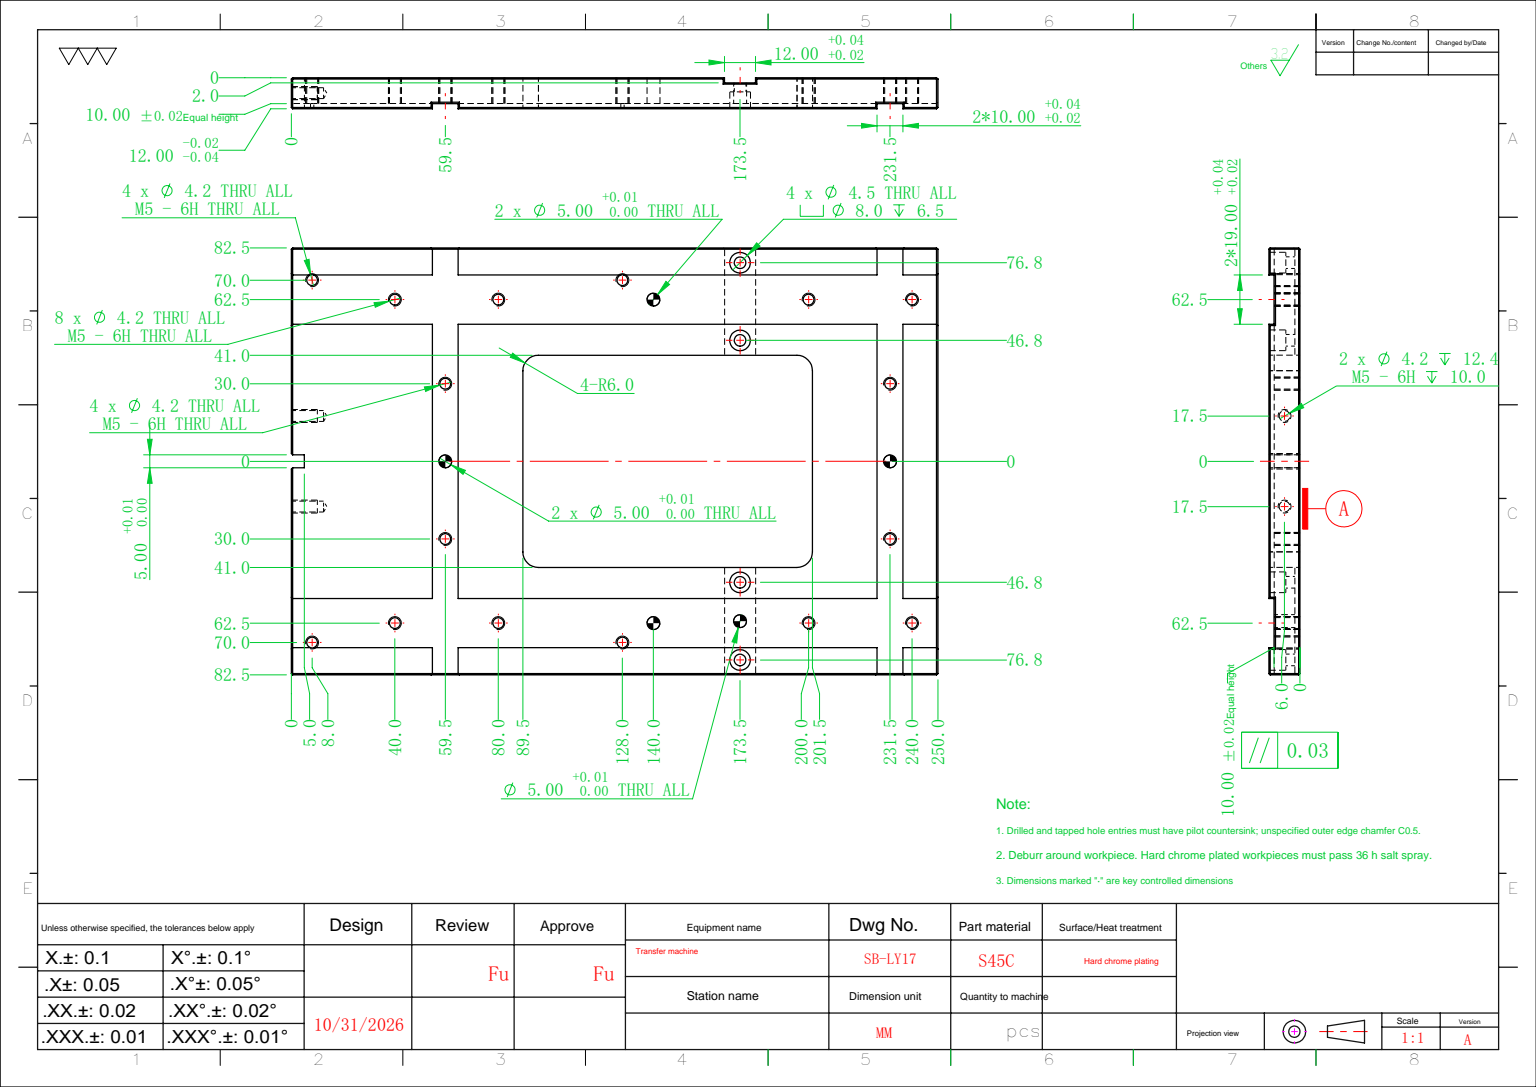
from build123d import *

# Parameters (mm, degrees)
SKETCH_1_W                   = 165
SKETCH_1_H                   = 250
EXTRUDE_1_DEPTH              = 12
SKETCH_2_W                   = 19
SKETCH_2_H                   = 250
CUT_EXTRUDE_1_DEPTH          = 2
SKETCH_3_W                   = 165
SKETCH_3_H                   = 10
CUT_EXTRUDE_2_DEPTH          = 2
SKETCH_4_W                   = 165
SKETCH_4_H                   = 10
CUT_EXTRUDE_3_DEPTH          = 2
HOLE_WIZARD_M5_1_D           = 4.2
MM_1_D                       = 5
CUT_EXTRUDE_4_DEPTH          = 151.250623959
SKETCH_11_W                  = 70
SKETCH_11_H                  = 112
CUT_EXTRUDE_5_DEPTH          = 151.250623959
SKETCH_13_W                  = 165
SKETCH_13_H                  = 12
CUT_EXTRUDE_6_DEPTH          = 2
HOLE_WIZARD_M5_2_D           = 4.2
HOLE_WIZARD_M4_1_D           = 4.5
HOLE_WIZARD_M4_1_CBORE_D     = 8
HOLE_WIZARD_M4_1_CBORE_DEPTH = 6.5
MM_2_D                       = 5
HOLE_WIZARD_M5_3_D           = 4.2
HOLE_WIZARD_M5_3_DEPTH       = 12.4
HOLE_WIZARD_M5_3_TIP         = 1.2618073
SKETCH_22_W                  = 5
SKETCH_22_H                  = 12
CUT_EXTRUDE_7_DEPTH          = 5
HOLE_WIZARD_M5_4_D           = 4.2
MM_3_D                       = 5
CHAMFER_1_SIZE               = 0.5


with BuildPart() as part:
    # 草图1 → 凸台-拉伸1 (new body)
    with BuildSketch(Plane.XY):
        Rectangle(SKETCH_1_W, SKETCH_1_H)
    extrude(amount=EXTRUDE_1_DEPTH)

    # 草图2 → 切除-拉伸1 (cut)
    with BuildSketch(Plane(origin=(0, 0, 0), x_dir=(-1, 0, 0), z_dir=(0, 0, -1))):
        with Locations((62.5, 0)):
            Rectangle(SKETCH_2_W, SKETCH_2_H)
        with Locations((-62.5, 0)):
            Rectangle(SKETCH_2_W, SKETCH_2_H)
    extrude(amount=-CUT_EXTRUDE_1_DEPTH, mode=Mode.SUBTRACT)

    # 草图3 → 切除-拉伸2 (cut)
    with BuildSketch(Plane(origin=(0, 0, 0), x_dir=(-1, 0, 0), z_dir=(0, 0, -1))):
        with Locations((0, -65.5)):
            Rectangle(SKETCH_3_W, SKETCH_3_H)
    extrude(amount=-CUT_EXTRUDE_2_DEPTH, mode=Mode.SUBTRACT)

    # 草图4 → 切除-拉伸3 (cut)
    with BuildSketch(Plane(origin=(0, 0, 0), x_dir=(-1, 0, 0), z_dir=(0, 0, -1))):
        with Locations((0, 106.5)):
            Rectangle(SKETCH_4_W, SKETCH_4_H)
    extrude(amount=-CUT_EXTRUDE_3_DEPTH, mode=Mode.SUBTRACT)

    # M5 螺纹孔1 (through all)
    with Locations(Plane(origin=(0, 0, 0), x_dir=(-1, 0, 0), z_dir=(0, 0, -1))):
        with Locations((-29.999242405, -65.5), (29.999242405, -65.5), (29.999242405, 106.5), (-29.999242405, 106.5)):
            Hole(HOLE_WIZARD_M5_1_D / 2)

    # 大小mm 暗销孔1 (through all)
    with Locations(Plane(origin=(0, 0, 2), x_dir=(-1, 0, 0), z_dir=(0, 0, -1))):
        with Locations((0, -65.5), (0, 106.5)):
            Hole(MM_1_D / 2)

    # 草图10 → 切除-拉伸4 (cut, through all)
    with BuildSketch(Plane(origin=(0, 0, 0), x_dir=(-1, 0, 0), z_dir=(0, 0, -1))):
        with BuildLine():
            Line((29, -29.5), (29, 70.5))
            ThreePointArc((29, 70.5), (35, 76.5), (41, 70.5))
            Line((41, 70.5), (41, -29.5))
            ThreePointArc((41, -29.5), (35, -35.5), (29, -29.5))
        make_face()
        with BuildLine():
            Line((-29, -29.5), (-29, 70.5))
            ThreePointArc((-29, 70.5), (-35, 76.5), (-41, 70.5))
            Line((-41, 70.5), (-41, -29.5))
            ThreePointArc((-41, -29.5), (-35, -35.5), (-29, -29.5))
        make_face()
    extrude(amount=-CUT_EXTRUDE_4_DEPTH, mode=Mode.SUBTRACT)

    # 草图11 → 切除-拉伸5 (cut, through all)
    with BuildSketch(Plane(origin=(0, 0, 0), x_dir=(-1, 0, 0), z_dir=(0, 0, -1))):
        with Locations((0, 20.5)):
            Rectangle(SKETCH_11_W, SKETCH_11_H)
    extrude(amount=-CUT_EXTRUDE_5_DEPTH, mode=Mode.SUBTRACT)

    # 草图13 → 切除-拉伸6 (cut)
    with BuildSketch(Plane.XY.offset(12)):
        with Locations((0, 48.5)):
            Rectangle(SKETCH_13_W, SKETCH_13_H)
    extrude(amount=-CUT_EXTRUDE_6_DEPTH, mode=Mode.SUBTRACT)

    # M5 螺纹孔2 (through all)
    with Locations(Plane.XY.offset(12)):
        with Locations((-70, 3), (-70, -117), (70, 3), (70, -117)):
            Hole(HOLE_WIZARD_M5_2_D / 2)

    # M4 六角凹头螺钉的柱形沉头孔1 (through all)
    with Locations(Plane(origin=(0, 0, 0), x_dir=(-1, 0, 0), z_dir=(0, 0, -1))):
        with Locations((46.75, 48.5), (76.75, 48.5), (-76.75, 48.5), (-46.75, 48.5)):
            CounterBoreHole(HOLE_WIZARD_M4_1_D / 2, HOLE_WIZARD_M4_1_CBORE_D / 2, HOLE_WIZARD_M4_1_CBORE_DEPTH)

    # 大小mm 暗销孔2 (through all)
    with Locations(Plane(origin=(0, 0, 2), x_dir=(-1, 0, 0), z_dir=(0, 0, -1))):
        with Locations((61.75, 48.5)):
            Hole(MM_2_D / 2)

    # M5 螺纹孔3
    with Locations(Plane(origin=(0, -125, 0), x_dir=(-1, 0, 0), z_dir=(0, -1, 0))):
        with Locations((-17.5, -6), (17.5, -6)):
            Hole(HOLE_WIZARD_M5_3_D / 2, depth=HOLE_WIZARD_M5_3_DEPTH)
            with Locations((0, 0, -(HOLE_WIZARD_M5_3_DEPTH + HOLE_WIZARD_M5_3_TIP / 2))):  # 118° drill point
                Cone(0, HOLE_WIZARD_M5_3_D / 2, HOLE_WIZARD_M5_3_TIP, mode=Mode.SUBTRACT)

    # 草图22 → 切除-拉伸7 (cut)
    with BuildSketch(Plane.XZ.offset(125)):
        with Locations((0, 6)):
            Rectangle(SKETCH_22_W, SKETCH_22_H)
    extrude(amount=-CUT_EXTRUDE_7_DEPTH, mode=Mode.SUBTRACT)

    # M5 螺纹孔4 (through all)
    with Locations(Plane(origin=(0, 0, 2), x_dir=(-1, 0, 0), z_dir=(0, 0, -1))):
        with Locations((62.5, -85), (62.5, -45), (62.5, 75), (62.5, 115), (-62.5, 115), (-62.5, 75), (-62.5, -45), (-62.5, -85)):
            Hole(HOLE_WIZARD_M5_4_D / 2)

    # 大小mm 暗销孔3 (through all)
    with Locations(Plane(origin=(0, 0, 2), x_dir=(-1, 0, 0), z_dir=(0, 0, -1))):
        with Locations((62.5, 15), (-62.5, 15)):
            Hole(MM_3_D / 2)

    # 倒角1
    chamfer_1_edges = [part.edges().sort_by_distance(p)[0] for p in [
        (82.5, 118.25, 0),
        (-82.5, 20.5, 0),
        (82.5, 111.5, 1),
        (-82.5, 101.5, 1),
        (82.5, 106.5, 2),
        (82.5, 101.5, 1),
        (-82.5, 106.5, 2),
        (-82.5, 111.5, 1),
        (-82.5, 89.75, 12),
        (-27.75, -125, 0),
        (77.25, -125, 0),
        (0, 125, 0),
        (-77.25, 125, 0),
        (-42.5, -125, 12),
        (-72, 125, 1),
        (-62.5, -125, 2),
        (-72, -125, 1),
        (-53, -125, 1),
        (-62.5, 125, 2),
        (-53, 125, 1),
        (82.5, 89.75, 12),
        (-82.5, -41.25, 12),
        (-82.5, 54.5, 11),
        (82.5, 42.5, 11),
        (-82.5, 48.5, 10),
        (-82.5, 42.5, 11),
        (82.5, 48.5, 10),
        (82.5, 54.5, 11),
        (62.5, 125, 2),
        (72, 125, 1),
        (53, 125, 1),
        (62.5, -125, 2),
        (53, -125, 1),
        (72, -125, 1),
        (27.75, -125, 0),
        (42.5, -125, 12),
        (-2.5, -125, 6),
        (2.5, -125, 6),
        (82.5, -41.25, 12),
        (-77.25, -125, 0),
        (-82.5, 118.25, 0),
        (82.5, 20.5, 0),
        (-82.5, -97.75, 0),
        (77.25, 125, 0),
        (82.5, -97.75, 0),
        (-82.5, -70.5, 1),
        (82.5, -60.5, 1),
        (-82.5, -65.5, 2),
        (-82.5, -60.5, 1),
        (82.5, -65.5, 2),
        (82.5, -70.5, 1),
        (82.5, -125, 6),
        (-82.5, -125, 6),
        (-82.5, 125, 6),
        (82.5, 125, 6),
        (0, 125, 12),
    ]]
    chamfer(chamfer_1_edges, length=CHAMFER_1_SIZE)


solid = part.part
